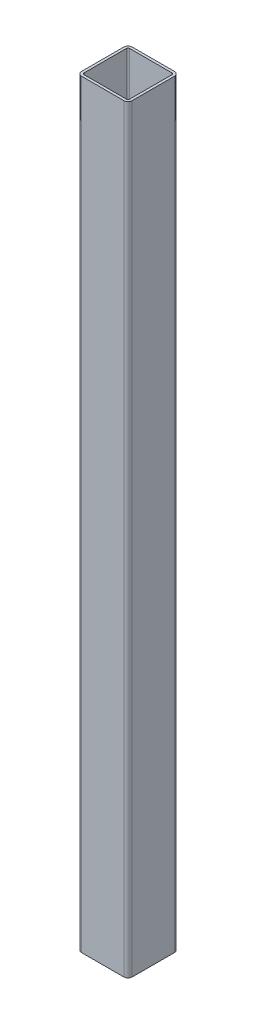
from build123d import *

# Parameters (mm, degrees)
BOSS_EXTRUDE1_DEPTH = 1800


with BuildPart() as part:
    # Sketch1 → Boss-Extrude1 (new body)
    with BuildSketch(Plane(origin=(0, 0, 0), x_dir=(1, 0, 0), z_dir=(0, 1, 0))):
        with BuildLine():
            Line((-50, -60), (50, -60))
            ThreePointArc((50, -60), (57.071067812, -57.071067812), (60, -50))
            Line((60, -50), (60, 50))
            ThreePointArc((60, 50), (57.071067812, 57.071067812), (50, 60))
            Line((50, 60), (-50, 60))
            ThreePointArc((-50, 60), (-57.071067812, 57.071067812), (-60, 50))
            Line((-60, 50), (-60, -50))
            ThreePointArc((-60, -50), (-57.071067812, -57.071067812), (-50, -60))
        make_face()
        with BuildLine():
            Line((-54, -50), (-54, 50))
            ThreePointArc((-54, 50), (-52.828427125, 52.828427125), (-50, 54))
            Line((-50, 54), (50, 54))
            ThreePointArc((50, 54), (52.828427125, 52.828427125), (54, 50))
            Line((54, 50), (54, -50))
            ThreePointArc((54, -50), (52.828427125, -52.828427125), (50, -54))
            Line((50, -54), (-50, -54))
            ThreePointArc((-50, -54), (-52.828427125, -52.828427125), (-54, -50))
        make_face(mode=Mode.SUBTRACT)
    extrude(amount=BOSS_EXTRUDE1_DEPTH)


solid = part.part
